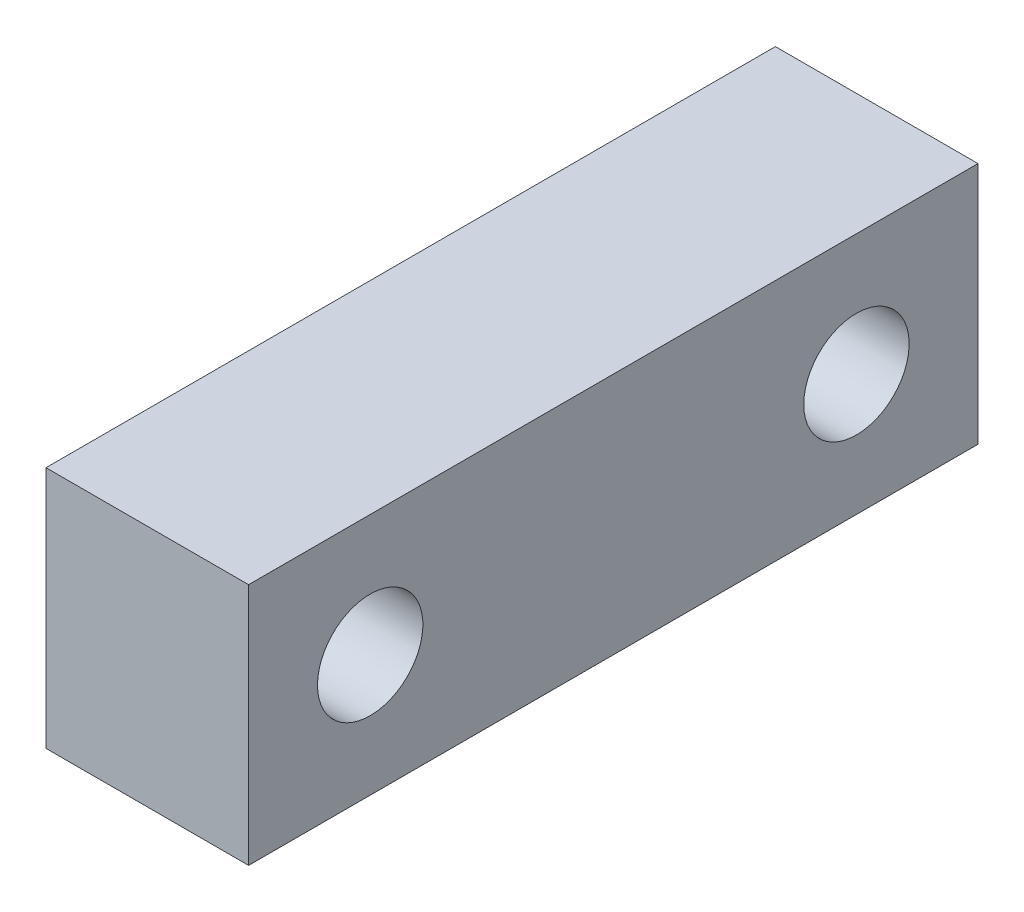
from build123d import *

# Parameters (mm, degrees)
SKETCH1_W           = 5
SKETCH1_H           = 18
BOSS_EXTRUDE1_DEPTH = 6
SKETCH2_R           = 1.3
CUT_EXTRUDE1_DEPTH  = 10
SKETCH3_R           = 2.3
CUT_EXTRUDE2_DEPTH  = 3


with BuildPart() as part:
    # Sketch1 → Boss-Extrude1 (new body)
    with BuildSketch(Plane(origin=(0, 0, 0), x_dir=(1, 0, 0), z_dir=(0, 1, 0))):
        Rectangle(SKETCH1_W, SKETCH1_H)
    extrude(amount=BOSS_EXTRUDE1_DEPTH)

    # Sketch2 → Cut-Extrude1 (cut)
    with BuildSketch(Plane.ZY.offset(2.5)):
        with Locations((6, 3)):
            Circle(SKETCH2_R)
        with Locations((-6, 3)):
            Circle(SKETCH2_R)
    extrude(amount=-CUT_EXTRUDE1_DEPTH, mode=Mode.SUBTRACT)

    # Sketch3 → Cut-Extrude2 (cut)
    with BuildSketch(Plane.ZY.offset(2.5)):
        with Locations((-6, 3)):
            Circle(SKETCH3_R)
        with Locations((6, 3)):
            Circle(SKETCH3_R)
    extrude(amount=-CUT_EXTRUDE2_DEPTH, mode=Mode.SUBTRACT)


solid = part.part
